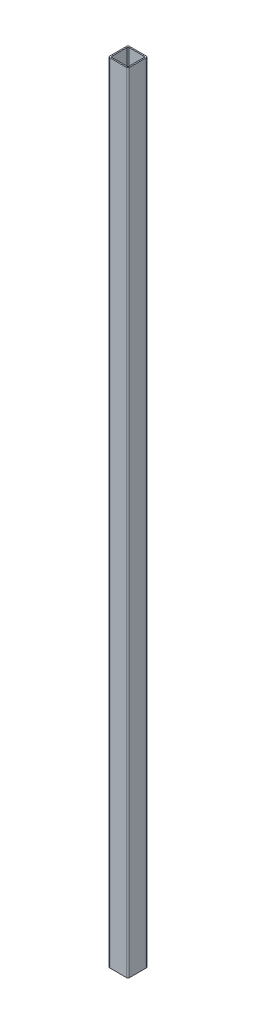
from build123d import *

# Parameters (mm, degrees)
BOSS_EXTRUDE1_DEPTH = 2000


with BuildPart() as part:
    # Sketch2 → Boss-Extrude1 (new, symmetric)
    with BuildSketch(Plane(origin=(0, 0, 0), x_dir=(1, 0, 0), z_dir=(0, 1, 0))):
        with BuildLine():
            Line((7.875, -1.525), (92.125, -1.525))
            ThreePointArc((92.125, -1.525), (97.693465902, 0.781534098), (100, 6.35))
            Line((100, 6.35), (100, 90.6))
            ThreePointArc((100, 90.6), (97.693465902, 96.168465902), (92.125, 98.475))
            Line((92.125, 98.475), (7.875, 98.475))
            ThreePointArc((7.875, 98.475), (2.306534098, 96.168465902), (0, 90.6))
            Line((0, 90.6), (0, 6.35))
            ThreePointArc((0, 6.35), (2.306534098, 0.781534098), (7.875, -1.525))
        make_face()
        with BuildLine():
            Line((12.6, 4.775), (87.4, 4.775))
            ThreePointArc((87.4, 4.775), (91.854772721, 6.620227279), (93.7, 11.075))
            Line((93.7, 11.075), (93.7, 85.875))
            ThreePointArc((93.7, 85.875), (91.854772721, 90.329772721), (87.4, 92.175))
            Line((87.4, 92.175), (12.6, 92.175))
            ThreePointArc((12.6, 92.175), (8.145227279, 90.329772721), (6.3, 85.875))
            Line((6.3, 85.875), (6.3, 11.075))
            ThreePointArc((6.3, 11.075), (8.145227279, 6.620227279), (12.6, 4.775))
        make_face(mode=Mode.SUBTRACT)
    extrude(amount=BOSS_EXTRUDE1_DEPTH, both=True)


solid = part.part
